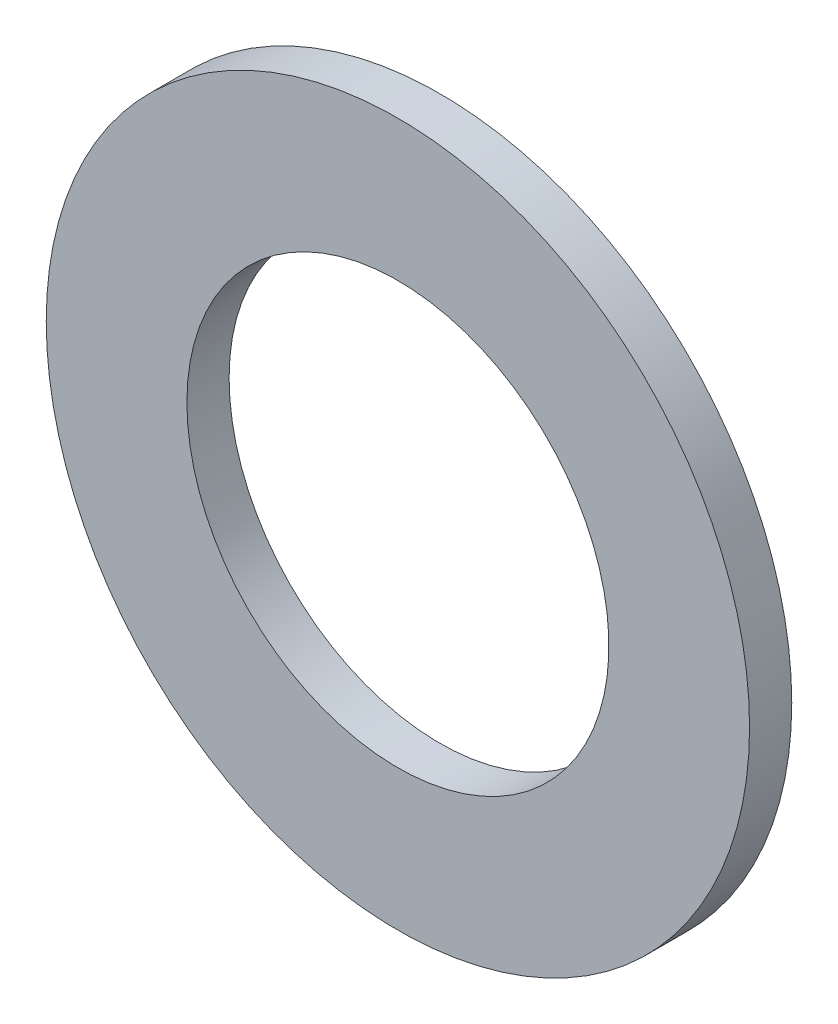
from build123d import *

# Parameters (mm, degrees)
SKETCH_1_R           = 2.5
BOSS_EXTRUDE_1_DEPTH = 0.3
SKETCH_2_R           = 1.5
CUT_EXTRUDE_1_DEPTH  = 0.3


with BuildPart() as part:
    # Sketch 1 → Boss-Extrude 1 (new body)
    with BuildSketch(Plane.XY):
        Circle(SKETCH_1_R)
    extrude(amount=BOSS_EXTRUDE_1_DEPTH)

    # Sketch 2 → Cut-Extrude 1 (cut)
    with BuildSketch(Plane(origin=(0, 0, 0), x_dir=(-1, 0, 0), z_dir=(0, 0, -1))):
        Circle(SKETCH_2_R)
    extrude(amount=-CUT_EXTRUDE_1_DEPTH, mode=Mode.SUBTRACT)


solid = part.part
